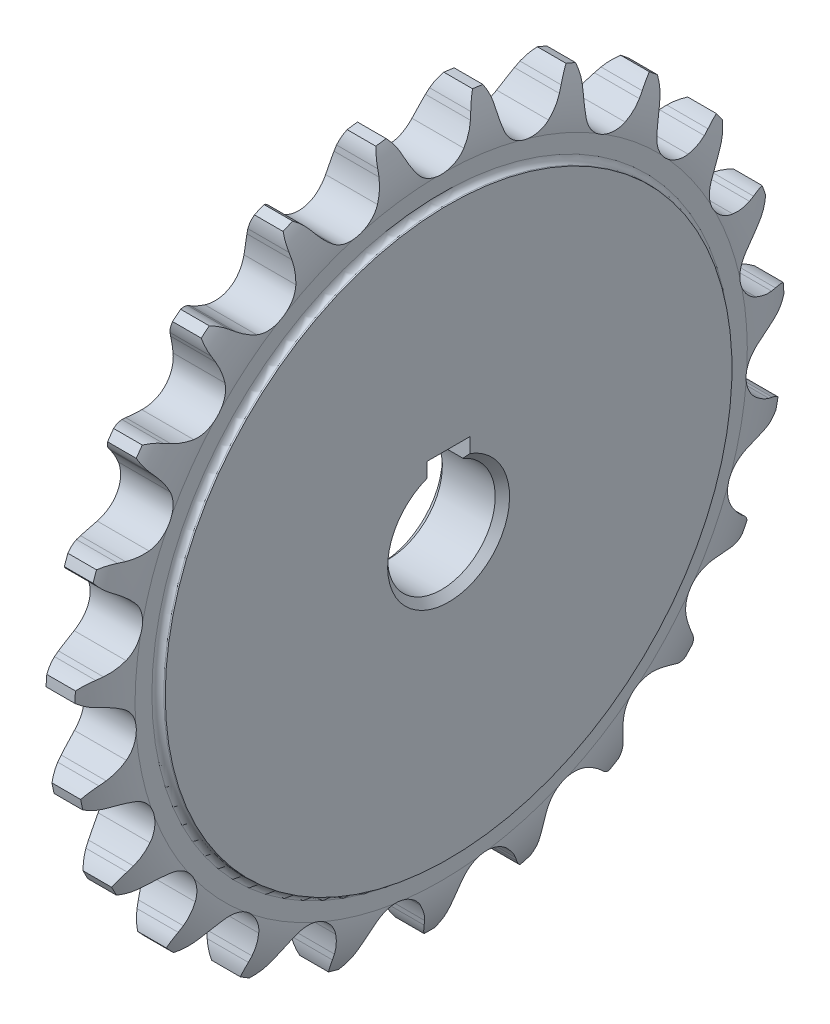
SolidWorks part; units mm, degrees
ref_plane "前视基准面" through (0, 0, 0) normal (0, 0, 1) x (1, 0, 0)
ref_plane "上视基准面" through (0, 0, 0) normal (0, 1, 0) x (1, 0, 0)
ref_plane "右视基准面" through (0, 0, 0) normal (1, 0, 0) x (0, 0, -1)
sketch "草图1" plane through (0, 0, 0) normal (0, 0, 1) x (1, 0, 0)
  line L0 (-6.35, 0) -> (6.35, 0) construction
  line L1 (-4.6852, 7.5) -> (-4.6852, 39.5)
  line L2 (-4.6852, 39.5) -> (-4.4782, 39.5)
  line L3 (-3.6502, 40.3279) -> (-3.6502, 42.674)
  line L4 (-1.9992, 49.5) -> (1.9992, 49.5)
  line L5 (3.6502, 42.674) -> (3.6502, 40.3279)
  line L6 (4.4782, 39.5) -> (4.6852, 39.5)
  line L7 (4.6852, 39.5) -> (4.6852, 7.5)
  line L8 (4.6852, 7.5) -> (-4.6852, 7.5)
  line L9 (0, 0) -> (0, 49.5) construction
  line L10 (-3.1938, 46.634) -> (3.1938, 46.634) construction
  line L11 (-3.1938, -46.634) -> (3.1938, -46.634) construction
  line L12 (6.35, 0) -> (29.35, 0) construction
  line L13 (-3.6502, 42.674) -> (3.7984, 42.674) construction
  line L14 (-3.6502, -42.674) -> (3.7984, -42.674) construction
  line L15 (29.35, 0) -> (37.27, 0) construction
  line L16 (37.27, 0) -> (49.34, 0) construction
  line L17 (49.34, 0) -> (57.19, 0) construction
  line L18 (57.19, 0) -> (71.57, 0) construction
  arc A0 (-1.9992, 49.5) -> (-3.6502, 42.674) centre (9.0381, 43.2177) ccw
  arc A1 (1.9992, 49.5) -> (3.6502, 42.674) centre (-9.0381, 43.2177) cw
  arc A2 (3.6502, 40.3279) -> (4.4782, 39.5) centre (4.4782, 40.3279) ccw
  arc A3 (-4.4782, 39.5) -> (-3.6502, 40.3279) centre (-4.4782, 40.3279) ccw
  point P30 (3.6502, 39.5)
  point P33 (-3.6502, 39.5)
  dimension "D1" = 3.174
  dimension "rx" = 12.7
  dimension "D3" = 0.8279
  dimension "d" = 93.2681
  dimension "p" = 12.7
  dimension "z" = 23
  dimension "da" = 99
  dimension "df" = 85.3481
  dimension "dr" = 7.92
  dimension "dk" = 15
  dimension "dg" = 79
  dimension "h" = 12.07
  dimension "bf1" = 7.3005
  dimension "b1" = 7.85
  dimension "ba" = 1.651
  dimension "D2" = 1.0349
  dimension "pt" = 14.38
revolve "旋转1" add sketch "草图1" angle 360 about L0
sketch "草图2" plane through (0, 0, 0) normal (1, 0, 0) x (0, 0, -1)
  line L0 (0, 0) -> (0, 49.5) construction
  line L1 (0, 0) -> (-6.7402, 49.039) construction
  line L2 (0, 0) -> (-13.3549, 47.6644) construction
  line L3 (3.1924, 44.1748) -> (7.0277, 41.2203) construction
  line L4 (4.5887, 46.6103) -> (-5.0194, 50.5007) construction
  line L5 (0, 0) -> (6.7402, 49.039) construction
  line L6 (4.5887, 46.6103) -> (4.8997, 47.3783)
  line L7 (-4.5887, 46.6103) -> (-4.8997, 47.3783)
  circle A0 centre (0, 0) radius 49.5 construction
  arc A1 (3.1924, 44.1748) -> (-3.1924, 44.1748) centre (0, 46.634) cw
  arc A2 (3.1924, 44.1748) -> (4.5887, 46.6103) centre (-5.0194, 50.5007) ccw
  arc A3 (6.0185, 49.1328) -> (4.8997, 47.3783) centre (10.2001, 45.2321) ccw
  arc A4 (-3.1924, 44.1748) -> (-4.5887, 46.6103) centre (5.0194, 50.5007) cw
  arc A5 (-6.0185, 49.1328) -> (-4.8997, 47.3783) centre (-10.2001, 45.2321) cw
  arc A7 (6.0185, 49.1328) -> (-6.0185, 49.1328) centre (0, 0) ccw
  dimension "r1" = 4.0298
  dimension "r3" = 5.7185
  dimension "D1" = 15.652
  dimension "D2" = 7.826
  dimension "α/2" = 52.391
  dimension "M" = 5.0194
  dimension "T" = 3.8666
  dimension "β" = 15.565
  dimension "γ/2" = 14.217
  dimension "bc" = 0.8285
extrude "切除-拉伸1" cut sketch "草图2" against normal mid plane 9.3703
pattern_circular "阵列(圆周)1" count 23 over 360 about axis through (0, 0, 0) along (1, 0, 0) of "切除-拉伸1"
sketch "草图3" plane through (0, 0, 0) normal (0, 0, 1) x (1, 0, 0)
  line L0 (4.6852, 7.5) -> (10.3148, 7.5)
  line L3 (10.3148, 7.5) -> (10.3148, 16.566)
  line L4 (10.3148, 16.566) -> (4.6852, 16.566)
  line L5 (4.6852, 16.566) -> (4.6852, 7.5)
  line L6 (0, 0) -> (4.8, 0) construction
  line L8 (-4.6852, 39.5) -> (-4.6852, -39.5) construction
  dimension "h" = 9.066
  dimension "K" = 4.8
  dimension "L" = 15
revolve "旋转2" [suppressed] add sketch "草图3" angle 360 about L6
sketch "草图4" plane through (-4.6852, 0, 0) normal (-1, 0, 0) x (0, 0, 1)
  line L1 (-3, 6.8739) -> (3, 6.8739)
  line L2 (-3, 6.8739) -> (-3, 10)
  line L3 (-3, 10) -> (3, 10)
  line L4 (3, 6.8739) -> (3, 10)
  circle A0 centre (0, 0) radius 7.5 construction
  point P6 (0.2, 10)
  dimension "D1" = 10
  dimension "键槽宽度" = 6
  dimension "t1" = 2.8
extrude "切除-拉伸2" cut sketch "草图4" against normal through all
chamfer "倒角1" distance 1 angle 45 1 edges at (-4.6852, -7.5, 0)
chamfer "倒角2" distance 1 angle 45 1 edges at (4.6852, -7.5, 0)
chamfer "倒角3" [suppressed] distance 1 angle 45
